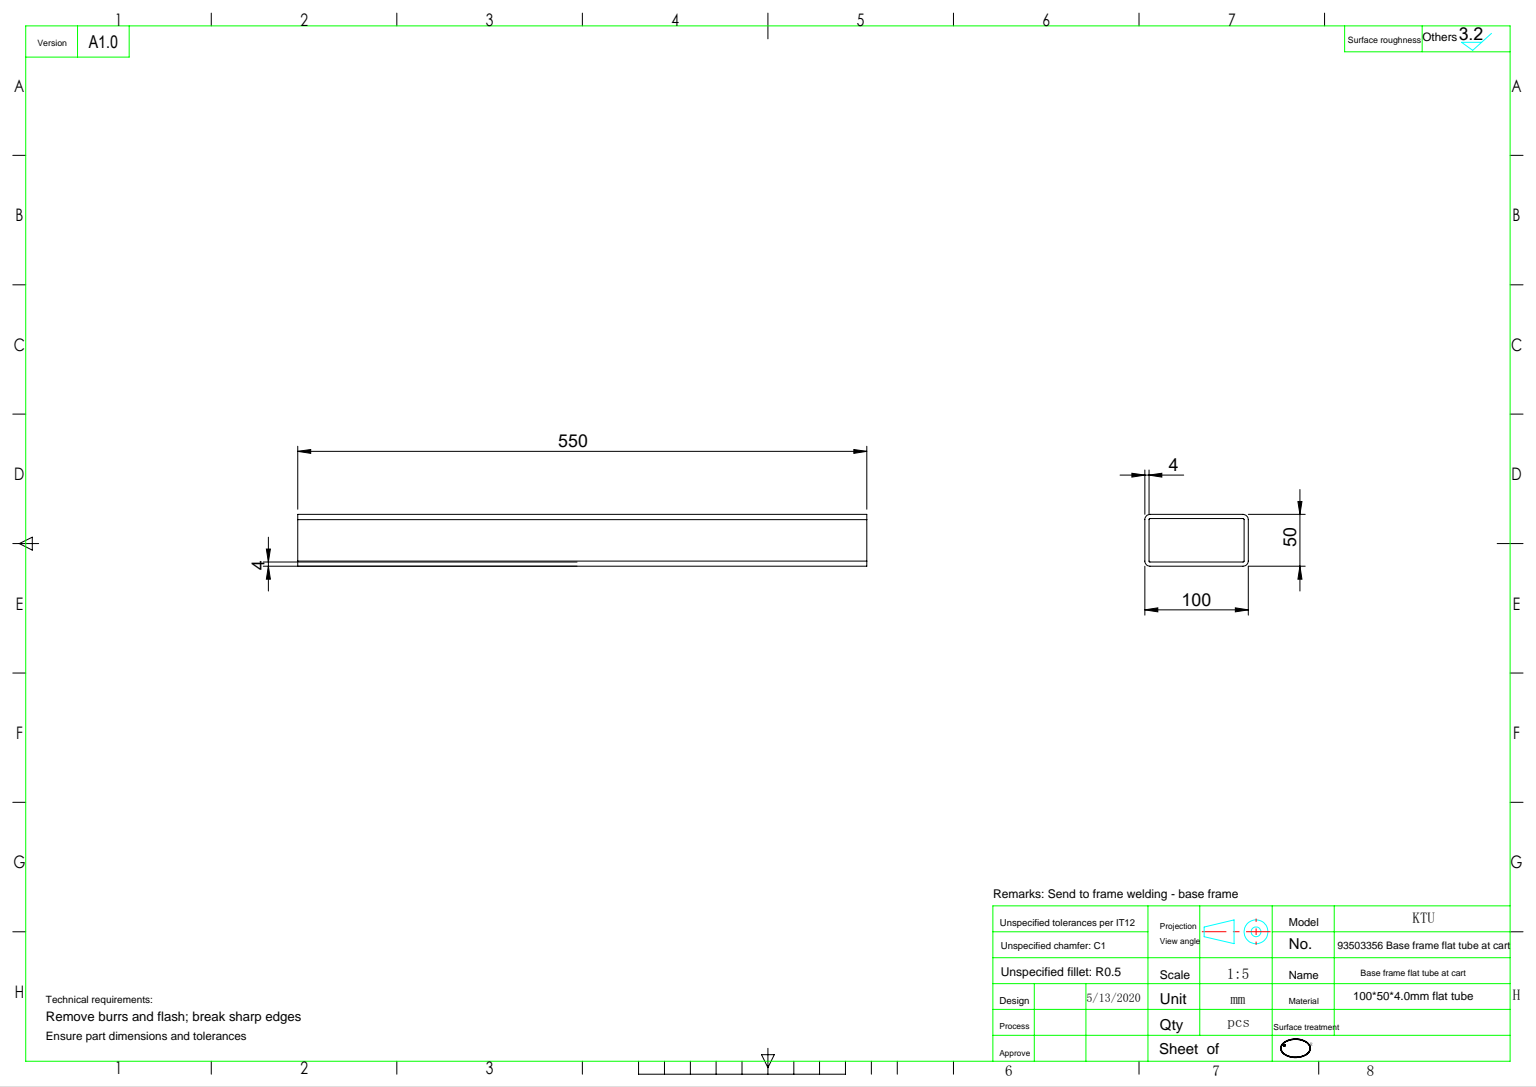
SolidWorks part; units mm, degrees
ref_plane "前视基准面" through (0, 0, 0) normal (0, 0, 1) x (1, 0, 0)
ref_plane "上视基准面" through (0, 0, 0) normal (0, 1, 0) x (1, 0, 0)
ref_plane "右视基准面" through (0, 0, 0) normal (1, 0, 0) x (0, 0, -1)
sketch "草图1" plane through (0, 0, 0) normal (0, 0, 1) x (1, 0, 0)
  line L1 (-45, 25) -> (45, 25)
  line L2 (-50, 20) -> (-50, -20)
  line L3 (-45, -25) -> (45, -25)
  line L4 (50, 20) -> (50, -20)
  line L5 (-50, 25) -> (50, -25) construction
  line L6 (-50, -25) -> (50, 25) construction
  arc A0 (45, -25) -> (50, -20) centre (45, -20) ccw
  arc A1 (45, 25) -> (50, 20) centre (45, 20) cw
  arc A2 (-50, -20) -> (-45, -25) centre (-45, -20) ccw
  arc A3 (-45, 25) -> (-50, 20) centre (-45, 20) ccw
  point P0 (0, 0)
  dimension "D3" = 5
  dimension "D1" = 100
  dimension "D2" = 50
extrude "拉伸-薄壁1" add sketch "草图1" along normal mid plane 550 thin
